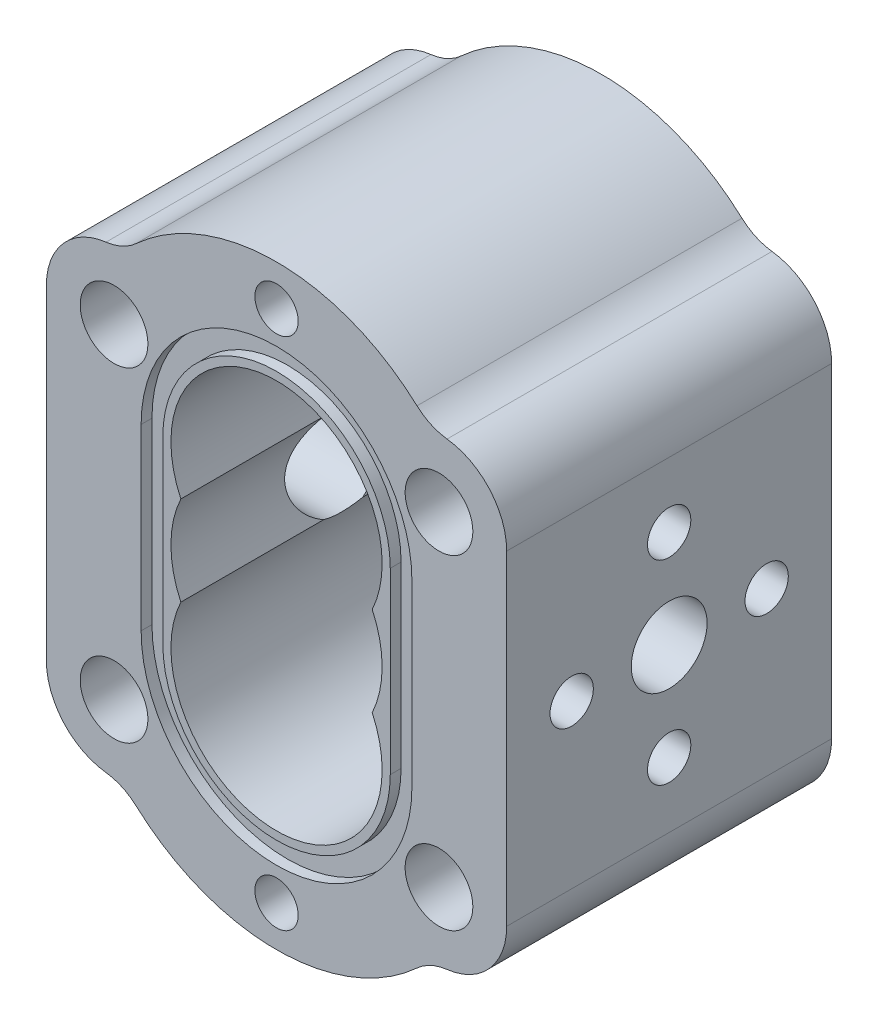
SolidWorks part; units mm, degrees
ref_plane "前视基准面" through (0, 0, 0) normal (0, 0, 1) x (1, 0, 0)
ref_plane "上视基准面" through (0, 0, 0) normal (0, 1, 0) x (1, 0, 0)
ref_plane "右视基准面" through (0, 0, 0) normal (1, 0, 0) x (0, 0, -1)
sketch "草图2" plane through (0, 0, 0) normal (0, 0, 1) x (1, 0, 0)
  line L0 (-7.133, 0) -> (11.209, 0) construction
  line L1 (-12.8551, 16.5) -> (14.8147, 16.5) construction
  line L2 (-16.9311, -16.5) -> (20.38, -16.5) construction
  line L3 (0, 22.7708) -> (0, 0) construction
  line L4 (0, -16.5) -> (0, -29.6686) construction
  line L5 (-42.5, 30) -> (-42.5, -30)
  line L6 (42.5, 30) -> (42.5, -30)
  line L7 (-30, 30) -> (30, 30) construction
  line L9 (-30, 30) -> (-30, -30) construction
  line L10 (-30, -30) -> (30, -30) construction
  line L11 (30, 30) -> (30, -30) construction
  line L13 (-16.5, -16.5) -> (0, 0) construction
  arc A0 (28.4793, 42.4072) -> (-28.4793, 42.4072) centre (0, 16.5) ccw
  arc A1 (28.4793, -42.4072) -> (-28.4793, -42.4072) centre (0, -16.5) cw
  arc A2 (-28.4793, 42.4072) -> (-42.5, 30) centre (-30, 30) ccw
  arc A4 (-42.5, -30) -> (-28.4793, -42.4072) centre (-30, -30) ccw
  arc A5 (28.4793, -42.4072) -> (42.5, -30) centre (30, -30) ccw
  arc A6 (42.5, 30) -> (28.4793, 42.4072) centre (30, 30) ccw
  point P15 (0, 0)
  dimension "D3" = 25
  dimension "D5" = 60
  dimension "D6" = 38.5
  dimension "D7" = 25
  dimension "D8" = 60
  dimension "D9" = 25
  dimension "D1" = 33
  dimension "D2" = 16.5
extrude "凸台-拉伸1" add sketch "草图2" along normal blind 60
sketch "草图3" plane through (0, 0, 60) normal (0, 0, 1) x (1, 0, 0)
  line L1 (-30, 30) -> (30, 30) construction
  line L2 (-30, 30) -> (-30, -30) construction
  line L3 (-30, -30) -> (30, -30) construction
  line L4 (30, 30) -> (30, -30) construction
  circle A0 centre (-30, 30) radius 6.25
  circle A1 centre (30, 30) radius 6.25
  circle A2 centre (-30, -30) radius 6.25
  circle A3 centre (30, -30) radius 6.25
  point P0 (0, 0)
  dimension "D3" = 12.5
  dimension "D4" = 12.5
  dimension "D1" = 60
  dimension "D2" = 60
extrude "切除-拉伸1" cut sketch "草图3" against normal through all
sketch "草图4" plane through (0, 0, 60) normal (0, 0, 1) x (1, 0, 0)
  arc A0 (17.6688, 8.25) -> (-17.6688, 8.25) centre (0, 16.5) ccw
  arc A1 (-17.6688, 8.25) -> (-17.6688, -8.25) centre (0, 0) ccw
  arc A2 (-17.6688, -8.25) -> (17.6688, -8.25) centre (0, -16.5) ccw
  arc A3 (17.6688, -8.25) -> (17.6688, 8.25) centre (0, 0) ccw
  dimension "D1" = 39
  dimension "D2" = 39
  dimension "D3" = 39
extrude "切除-拉伸2" cut sketch "草图4" against normal through all
sketch "草图5" plane through (0, 0, 60) normal (0, 0, 1) x (1, 0, 0)
  line L0 (-21, 16.5) -> (-21, -16.5)
  line L1 (-25, 16.5) -> (-25, -16.5)
  line L2 (21, 16.5) -> (21, -16.5)
  line L3 (25, 16.5) -> (25, -16.5)
  arc A0 (21, 16.5) -> (-21, 16.5) centre (0, 16.5) ccw
  arc A1 (-21, -16.5) -> (21, -16.5) centre (0, -16.5) ccw
  arc A2 (25, 16.5) -> (-25, 16.5) centre (0, 16.5) ccw
  arc A3 (-25, -16.5) -> (25, -16.5) centre (0, -16.5) ccw
  dimension "D1" = 42
  dimension "D2" = 42
  dimension "D3" = 4
extrude "切除-拉伸3" cut sketch "草图5" against normal blind 2
sketch "草图6" plane through (0, 0, 60) normal (0, 0, 1) x (1, 0, 0)
  line L0 (0, 59.2718) -> (0, -62.9833) construction
  circle A0 centre (0, 47.5) radius 4
  circle A1 centre (0, -47.5) radius 4
  dimension "D1" = 8
  dimension "D2" = 8
  dimension "D3" = 47.5
  dimension "D4" = 47.5
extrude "切除-拉伸4" cut sketch "草图6" against normal blind 6
ref_plane "基准面1" through (0, 0, 30) normal (0, 0, 1) x (1, 0, 0)
mirror "镜向1" about plane through (0, 0, 30) normal (0, 0, 1) of "切除-拉伸3"
sketch "草图7" plane through (43, 0, 0) normal (1, 0, 0) x (0, 0, -1)
  line L0 (7.0573, 0) -> (-71.5899, 0) construction
  line L1 (-30, 30) -> (-30, -30) construction
  line L2 (-60, 30) -> (0, 30) construction
  line L3 (-60, -30) -> (0, -30) construction
  circle A0 centre (-30, 0) radius 18 construction
  circle A1 centre (-30, 18) radius 4
  circle A2 centre (-48, 0) radius 4
  circle A3 centre (-30, -18) radius 4
  circle A4 centre (-12, 0) radius 4
  point P19 (0, 0)
  dimension "D2" = 8
  dimension "D3" = 8
  dimension "D1" = 36
  dimension "D4" = 8
  dimension "D5" = 8
sketch "草图10" plane through (43, 0, 0) normal (1, 0, 0) x (0, 0, -1)
  circle A0 centre (-30, 0) radius 7
  dimension "D1" = 14
extrude "切除-拉伸5" cut sketch "草图10" against normal up to next
sketch "草图11" plane through (-43, 0, 0) normal (-1, 0, 0) x (0, 0, 1)
  circle A0 centre (30, 0) radius 9
  dimension "D1" = 18
extrude "切除-拉伸6" cut sketch "草图11" against normal up to next
extrude "切除-拉伸7" cut sketch "草图7" against normal blind 15
mirror "镜向2" about plane through (0, 0, 0) normal (1, 0, 0) of "切除-拉伸7"
fillet "圆角1" radius 10 4 edges at (28.4793, -42.4072, 30) (-28.4793, -42.4072, 30) (28.4793, 42.4072, 30) (-28.4793, 42.4072, 30)
